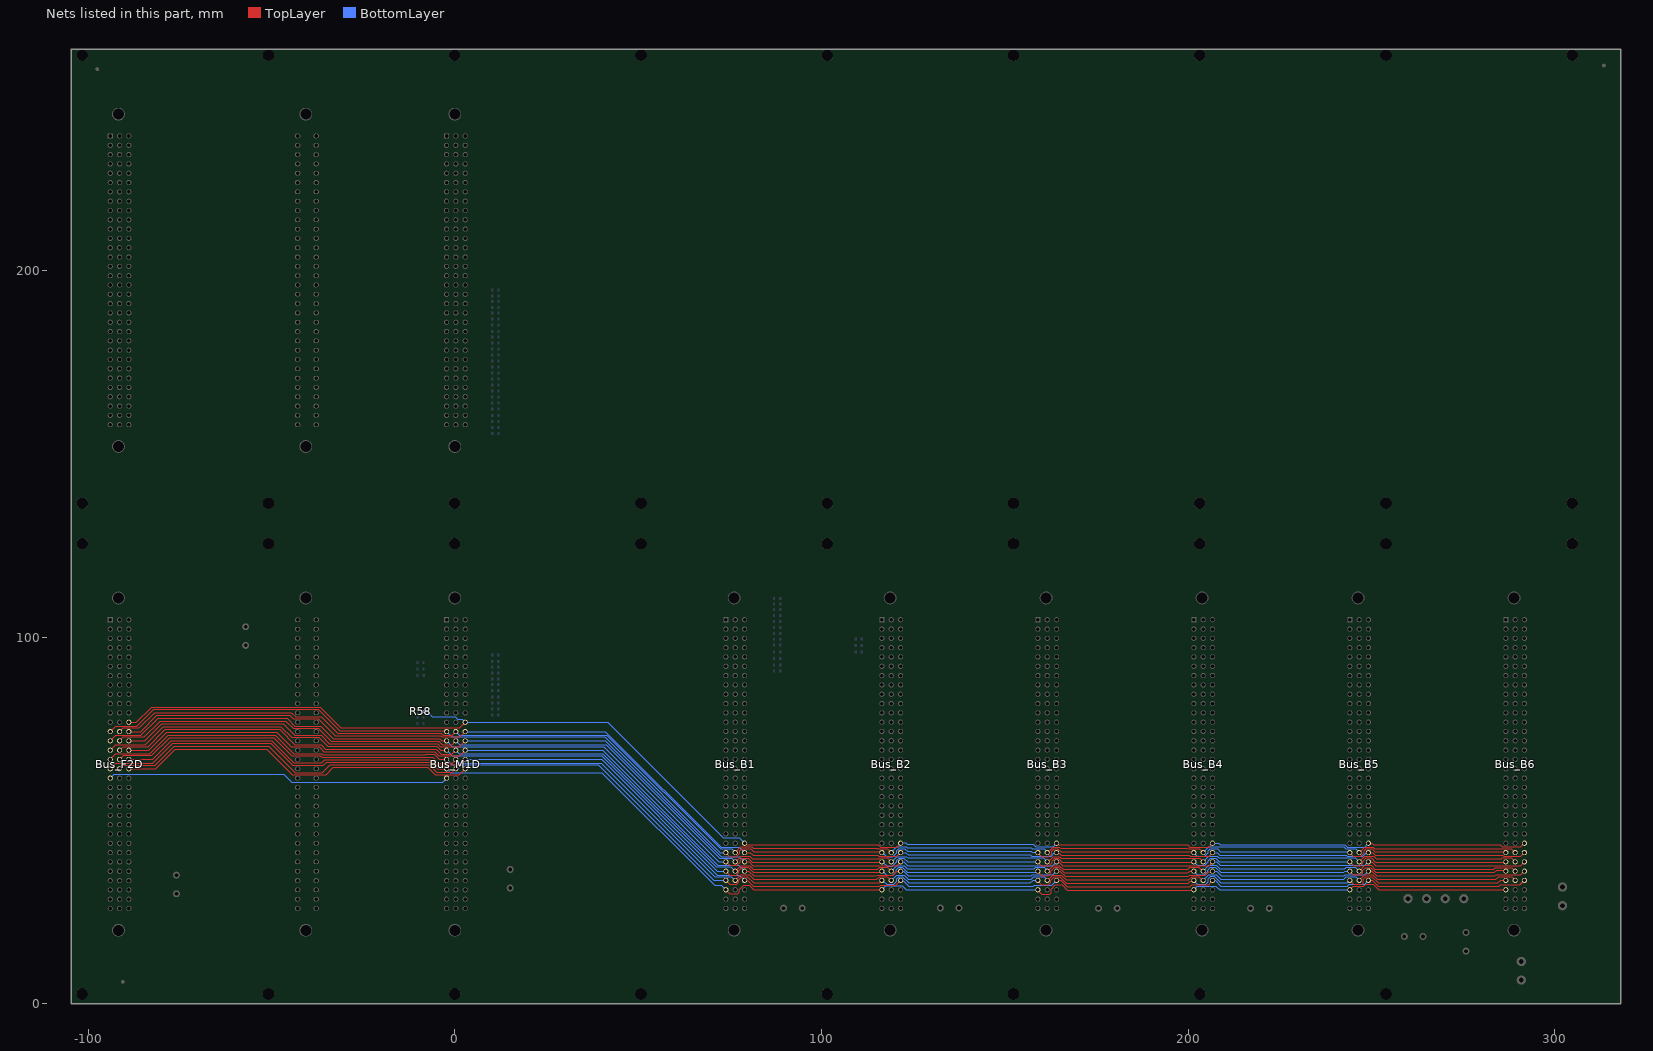
[diagram p0: the nets of this part, all layers, seen from the top]
# Altium PCB MISC67337.PcbDoc (part 2 of 7)
Units mm, origin at the board's own origin, x right, y up, seen from the top; angles counter-clockwise.
Board outline 422.71 x 260.35 mm, 4 copper layers (TopLayer, InternalPlane1, InternalPlane2, BottomLayer); 82 components, 143 nets, 1295 pads, 42 vias.

## Via types
v1: diameter 0.61, hole 0.305, TopLayer to BottomLayer, 42 vias

## Nets (pads, with @x,y where several pads share a name; then routed paths per layer and width w, separated by ;. In a path a pad name is that pad's centre, name@x,y a point inside that pad or via, vN(x,y) a via of type N, cw(c..) or ccw(c..) an arc to the next point about the centre after c; other vN are vias at no path point) (continued)
B_DSP1_X\W\E\: Bus_B1.C25 Bus_B2.C25 Bus_B3.C25 Bus_B4.C25 Bus_B5.C25 Bus_B6.C25 Bus_F2D.C12 Bus_M1D.C12 R58.2 | length 420.3
  TopLayer w0.254: Bus_F2D.C12@-88.89,76.754 -86.822,76.754 -82.68,80.896 -36.7,80.896 -31.039,75.235 1.321,75.235 Bus_M1D.C12@2.84,76.754 ; Bus_B1.C25@79.04,43.324 113.233,43.324 ; 113.727,43.324 113.233,43.324 ; Bus_B2.C25@121.521,43.817 Bus_B2.C25@121.585,43.88 ; Bus_B2.C25@121.585,43.753 120.504,42.672 116.203,42.672 115.551,43.324 113.233,43.324 ; Bus_B3.C25@164.13,43.308 198.425,43.308 ; 198.817,43.308 198.425,43.308 ; Bus_B4.C25@206.675,43.753 205.594,42.672 200.533,42.672 199.897,43.308 198.425,43.308 ; Bus_B5.C25@249.409,43.942 Bus_B5.C25@249.22,43.753 250.176,43.753 250.605,43.324 284.226,43.324 ; 284.607,43.324 284.226,43.324 ; Bus_B6.C25@291.765,43.753 290.787,42.775 285.774,42.775 285.225,43.324 284.226,43.324
  BottomLayer w0.254: R58.2@-8.484,79.705 -7.569,79.705 -6.18,78.316 0.121,78.316 0.84,77.597 1.997,77.597 Bus_M1D.C12@2.84,76.754 41.737,76.754 73.279,45.212 77.576,45.212 Bus_B1.C25@79.035,43.753 ; Bus_B2.C25@121.585,43.753 121.647,43.815 122.961,43.815 123.369,43.408 125.578,43.408 ; 124.93,43.408 125.578,43.408 ; 151.892,43.408 151.308,43.408 ; Bus_B3.C25@164.257,43.815 163.176,42.734 158.496,42.734 157.822,43.408 151.308,43.408 ; Bus_B4.C25@206.675,43.753 208.407,43.753 208.778,43.382 211.074,43.382 ; 209.893,43.382 211.074,43.382 ; 236.855,43.382 236.296,43.382 ; Bus_B5.C25@249.22,43.753 248.139,42.672 243.459,42.672 242.749,43.382 236.296,43.382 ; 125.578,43.408 151.308,43.408 ; 211.074,43.382 236.296,43.382
B_DSP1_XA0: Bus_B1.A26 Bus_B2.A26 Bus_B3.A26 Bus_B4.A26 Bus_B5.A26 Bus_B6.A26 Bus_F2D.A13 Bus_M1D.A13 | length 414.4
  TopLayer w0.254: Bus_F2D.A13@-93.97,74.214 -92.492,75.692 -86.69,75.692 -82.118,80.264 -37.236,80.264 -31.411,74.438 Bus_M1D.A13@-2.6,74.438 ; Bus_M1D.A13@-2.6,74.574 Bus_M1D.A13@-2.24,74.214 ; Bus_B1.A26@73.96,41.213 75.041,40.132 76.835,40.132 77.724,41.021 77.724,41.656 78.259,42.191 80.779,42.191 81.534,41.436 112.243,41.436 ; 113.349,41.436 112.243,41.436 ; Bus_B2.A26@116.505,41.213 Bus_B2.A26@116.378,41.34 ; Bus_B2.A26@116.505,41.34 Bus_B2.A26@116.378,41.34 ; Bus_B3.A26@159.05,41.086 160.131,40.005 161.925,40.005 162.814,40.894 162.814,41.529 163.576,42.291 164.491,42.291 165.379,41.403 197.993,41.403 ; 198.439,41.403 197.993,41.403 ; Bus_B4.A26@201.595,41.086 201.468,41.213 Bus_B4.A26@201.595,41.213 201.405,41.403 197.993,41.403 ; Bus_B5.A26@244.14,41.213 245.118,40.235 247.118,40.235 248.031,41.148 248.031,41.656 248.566,42.191 250.188,42.191 250.943,41.436 286.462,41.436 Bus_B6.A26@286.685,41.213 ; 112.243,41.436 116.282,41.436 Bus_B2.A26@116.378,41.34
  BottomLayer w0.254: Bus_M1D.A13@-2.24,74.214 -0.797,72.771 40.894,72.771 72.452,41.213 Bus_B1.A26@73.955,41.213 ; Bus_B2.A26@116.632,41.275 117.775,40.132 119.445,40.132 120.523,41.21 120.523,41.718 121.071,42.266 122.758,42.266 123.517,41.507 154.584,41.507 ; 156.424,41.507 154.584,41.507 ; Bus_B3.A26@159.177,41.275 157.415,41.275 157.183,41.507 154.584,41.507 ; Bus_B4.A26@201.595,41.213 202.573,40.235 204.573,40.235 205.486,41.148 205.486,41.656 206.045,42.215 208.077,42.215 208.807,41.485 240.208,41.485 ; 241.222,41.485 240.208,41.485 ; Bus_B5.A26@244.14,41.213 243.868,41.485 240.208,41.485
B_DSP1_XA1: Bus_B1.B26 Bus_B2.B26 Bus_B3.B26 Bus_B4.B26 Bus_B5.B26 Bus_B6.B26 Bus_F2D.B13 Bus_M1D.B13 | length 408.8
  TopLayer w0.254: Bus_F2D.B13@-91.43,74.214 -90.452,75.192 -85.996,75.192 -81.819,79.369 -44.571,79.369 -43.434,78.232 -36.449,78.232 -31.941,73.724 -3.632,73.724 -3.144,73.236 -0.678,73.236 Bus_M1D.B13@0.3,74.214 ; Bus_B1.B26@76.495,41.213 78.057,42.775 80.961,42.775 81.356,42.38 115.328,42.38 115.443,42.266 ; 115.418,42.266 115.443,42.266 ; Bus_B2.B26@119.045,41.213 117.992,42.266 115.443,42.266 ; Bus_B3.B26@161.59,41.086 163.201,42.697 164.885,42.697 165.227,42.355 198.857,42.355 ; 199.011,42.355 198.857,42.355 ; Bus_B4.B26@204.135,41.086 203.03,42.191 199.998,42.191 199.834,42.355 198.857,42.355 ; Bus_B5.B26@246.68,41.213 246.699,41.213 248.158,42.672 250.508,42.672 250.889,42.291 285.826,42.291 ; 285.115,42.291 285.826,42.291 ; Bus_B6.B26@289.225,41.213 288.147,42.291 285.826,42.291
  BottomLayer w0.254: Bus_M1D.B13@0.3,74.214 1.278,73.236 41.443,73.236 72.488,42.191 75.517,42.191 Bus_B1.B26@76.495,41.213 ; Bus_B2.B26@119.045,41.213 120.58,42.748 123.178,42.748 123.469,42.457 125.527,42.457 155.169,42.457 ; 157.161,42.457 155.169,42.457 ; Bus_B3.B26@161.717,41.275 160.739,42.253 157.493,42.253 157.288,42.457 155.169,42.457 ; Bus_B4.B26@204.135,41.213 205.67,42.748 242.494,42.748 243.051,42.191 245.702,42.191 Bus_B5.B26@246.68,41.213
B_DSP1_XA2: Bus_B1.C26 Bus_B2.C26 Bus_B3.C26 Bus_B4.C26 Bus_B5.C26 Bus_B6.C26 Bus_F2D.C13 Bus_M1D.C13 | length 408.7
  TopLayer w0.254: Bus_F2D.C13@-88.89,74.214 -85.704,74.214 -81.313,78.606 -45.027,78.606 -44.09,77.668 -37.257,77.668 -32.599,73.01 -6.096,73.01 ; -3.835,73.01 -6.096,73.01 ; Bus_M1D.C13@2.84,74.214 1.397,72.771 -3.581,72.771 -3.82,73.01 -6.096,73.01 ; Bus_B1.C26@79.035,41.213 Bus_B1.C26@79.04,41.213 ; Bus_B1.C26@79.229,41.402 Bus_B1.C26@79.04,41.213 ; Bus_B2.C26@121.585,41.213 120.529,40.157 115.672,40.157 115.337,40.492 81.377,40.492 80.656,41.213 Bus_B1.C26@79.04,41.213 ; Bus_B3.C26@164.13,41.086 Bus_B3.C26@164.193,41.15 ; Bus_B3.C26@164.13,41.213 Bus_B3.C26@164.193,41.15 ; Bus_B3.C26@164.319,41.275 Bus_B3.C26@164.193,41.15 ; Bus_B4.C26@206.675,41.086 205.746,40.157 200.635,40.157 200.342,40.45 165.467,40.45 164.768,41.15 Bus_B3.C26@164.193,41.15 ; Bus_B5.C26@249.22,41.213 250.404,41.213 251.125,40.492 283.718,40.492 ; 284.034,40.492 283.718,40.492 ; 286.106,40.235 286.131,40.235 ; Bus_B6.C26@291.765,41.213 290.787,40.235 286.131,40.235 ; 283.718,40.492 285.874,40.492 286.131,40.235
  BottomLayer w0.254: Bus_M1D.C13@2.84,74.214 41.102,74.214 72.644,42.672 77.576,42.672 Bus_B1.C26@79.035,41.213 ; Bus_B2.C26@121.585,41.213 123.023,41.213 123.68,40.557 155.6,40.557 ; 156.272,40.557 155.6,40.557 ; Bus_B3.C26@164.257,41.275 163.673,41.275 162.631,40.234 157.313,40.234 156.99,40.557 155.6,40.557 ; Bus_B4.C26@206.675,41.213 208.012,41.213 208.688,40.537 239.776,40.537 ; 241.235,40.537 239.776,40.537 ; Bus_B5.C26@249.22,41.213 248.636,41.213 247.658,40.235 243.434,40.235 243.132,40.537 239.776,40.537
B_DSP1_XA3: Bus_B1.A27 Bus_B2.A27 Bus_B3.A27 Bus_B4.A27 Bus_B5.A27 Bus_B6.A27 Bus_F2D.A14 Bus_M1D.A14 | length 415.5
  TopLayer w0.254: Bus_F2D.A14@-93.97,71.674 -92.492,73.152 -85.623,73.152 -80.933,77.842 -45.736,77.842 -43.586,75.692 -36.601,75.692 -33.205,72.296 -6.426,72.296 ; -4.496,72.296 -6.426,72.296 ; Bus_M1D.A14@-2.24,71.674 -3.526,71.674 -4.148,72.296 -6.426,72.296 ; Bus_B1.A27@73.96,38.673 74.938,37.695 76.938,37.695 77.851,38.608 77.851,39.116 78.386,39.651 80.085,39.651 81.131,38.604 113.665,38.604 ; 113.944,38.604 113.665,38.604 ; Bus_B2.A27@116.505,38.673 116.436,38.604 113.665,38.604 ; Bus_B3.A27@159.05,38.546 160.028,37.568 162.028,37.568 162.941,38.481 162.941,38.989 163.603,39.651 164.641,39.651 165.747,38.546 198.069,38.546 ; 198.982,38.546 198.069,38.546 ; Bus_B4.A27@201.595,38.673 201.468,38.546 198.069,38.546 ; Bus_B5.A27@244.14,38.673 245.221,37.592 246.982,37.592 247.658,38.268 247.658,38.743 248.666,39.751 249.911,39.751 251.057,38.604 282.372,38.604 ; 283.34,38.604 282.372,38.604 ; Bus_B6.A27@286.685,38.673 286.616,38.604 282.372,38.604
  BottomLayer w0.254: Bus_M1D.A14@-2.24,71.674 -0.678,70.112 40.632,70.112 72.071,38.673 Bus_B1.A27@73.955,38.673 ; Bus_B2.A27@116.632,38.735 117.902,37.465 119.285,37.465 120.523,38.703 120.523,39.051 121.185,39.713 122.466,39.713 123.523,38.656 154.965,38.656 ; 155.929,38.656 154.965,38.656 ; Bus_B3.A27@159.05,38.673 159.033,38.656 154.965,38.656 ; Bus_B3.A27@159.05,38.735 Bus_B3.A27@159.177,38.735 ; Bus_B4.A27@201.595,38.673 202.573,37.695 204.54,37.695 205.486,38.641 205.486,38.989 206.148,39.651 207.567,39.651 208.578,38.64 240.005,38.64 ; 240.892,38.64 240.005,38.64 ; Bus_B5.A27@244.14,38.673 244.107,38.64 240.005,38.64
B_DSP1_XA4: Bus_B1.B27 Bus_B2.B27 Bus_B3.B27 Bus_B4.B27 Bus_B5.B27 Bus_B6.B27 Bus_F2D.B14 Bus_M1D.B14 | length 412.5
  TopLayer w0.254: Bus_F2D.B14@-91.43,71.674 -90.358,72.746 -84.684,72.746 -80.351,77.079 -46.065,77.079 -44.115,75.128 -37.232,75.128 -33.685,71.582 -29.642,71.582 ; -32.36,71.582 -29.642,71.582 ; -4.75,71.582 -5.817,71.582 ; Bus_M1D.B14@0.3,71.674 -0.751,70.623 -3.39,70.623 -4.348,71.582 -5.817,71.582 ; Bus_B1.B27@76.5,38.673 76.519,38.673 78.08,40.234 80.493,40.234 81.178,39.548 ; 81.153,39.548 81.178,39.548 ; 114.554,39.548 113.487,39.548 ; Bus_B2.B27@119.045,38.673 117.967,39.751 116.078,39.751 115.875,39.548 113.487,39.548 ; Bus_B3.B27@161.59,38.546 161.609,38.546 163.195,40.132 164.973,40.132 165.454,39.651 203.157,39.651 Bus_B4.B27@204.135,38.673 ; Bus_B4.B27@204.071,38.61 Bus_B4.B27@204.135,38.546 ; Bus_B5.B27@246.68,38.673 248.164,40.157 250.698,40.157 251.307,39.548 253.39,39.548 ; 252.425,39.548 253.39,39.548 ; 283.718,39.548 283.312,39.548 ; Bus_B6.B27@289.225,38.673 288.147,39.751 285.75,39.751 285.547,39.548 283.312,39.548 ; -29.642,71.582 -5.817,71.582 ; 81.178,39.548 113.487,39.548 ; 253.39,39.548 283.312,39.548
  BottomLayer w0.254: Bus_M1D.B14@0.3,71.674 1.362,70.612 41.275,70.612 72.236,39.651 75.517,39.651 Bus_B1.B27@76.495,38.673 ; Bus_B2.B27@119.172,38.735 120.569,40.132 123.139,40.132 123.546,39.726 160.537,39.726 Bus_B3.B27@161.59,38.673 ; Bus_B3.B27@161.684,38.768 Bus_B3.B27@161.717,38.735 ; Bus_B4.B27@204.135,38.673 205.645,40.183 207.924,40.183 208.356,39.751 245.602,39.751 Bus_B5.B27@246.68,38.673
B_DSP1_XA5: Bus_B1.C27 Bus_B2.C27 Bus_B3.C27 Bus_B4.C27 Bus_B5.C27 Bus_B6.C27 Bus_F2D.C14 Bus_M1D.C14 | length 410.1
  TopLayer w0.254: Bus_F2D.C14@-88.89,71.674 -84.557,71.674 -79.929,76.302 ; -79.929,76.315 -46.749,76.315 -43.586,73.152 -36.474,73.152 -34.19,70.867 -32.36,70.867 ; -33.249,70.867 -32.36,70.867 ; -5.174,70.867 -5.664,70.867 ; Bus_M1D.C14@2.84,71.674 1.278,70.112 -3.937,70.112 -4.693,70.867 -5.664,70.867 ; Bus_B1.C27@79.035,38.673 Bus_B1.C27@79.04,38.673 ; Bus_B1.C27@79.356,38.989 Bus_B1.C27@79.04,38.673 ; 113.538,37.661 112.674,37.661 ; Bus_B2.C27@121.585,38.673 120.573,37.661 112.674,37.661 ; Bus_B3.C27@164.13,38.546 Bus_B3.C27@164.257,38.673 ; Bus_B3.C27@164.13,38.673 Bus_B3.C27@164.257,38.673 ; Bus_B3.C27@164.446,38.862 Bus_B3.C27@164.257,38.673 ; 198.628,37.593 198.095,37.593 ; 199.873,37.617 200.99,37.617 ; Bus_B4.C27@206.675,38.546 205.746,37.617 200.99,37.617 ; Bus_B5.C27@249.22,38.673 250.125,38.673 251.137,37.661 282.448,37.661 ; 282.829,37.661 282.448,37.661 ; Bus_B6.C27@291.765,38.673 290.753,37.661 282.448,37.661 ; -32.36,70.867 -5.664,70.867 ; Bus_B1.C27@79.04,38.673 80.301,38.673 81.313,37.661 112.674,37.661 ; Bus_B3.C27@164.257,38.673 164.73,38.673 165.81,37.593 198.095,37.593 ; 198.095,37.593 198.119,37.617 200.99,37.617
  BottomLayer w0.254: Bus_M1D.C14@2.84,71.674 41.102,71.674 72.644,40.132 77.576,40.132 Bus_B1.C27@79.035,38.673 ; Bus_B2.C27@121.585,38.673 122.515,38.673 123.546,37.643 163.1,37.643 Bus_B3.C27@164.13,38.673 ; Bus_B3.C27@164.163,38.641 Bus_B3.C27@164.257,38.735 ; Bus_B4.C27@206.675,38.673 207.783,38.673 208.765,37.691 239.573,37.691 ; 240.73,37.691 239.573,37.691 ; Bus_B5.C27@249.22,38.673 248.238,37.691 239.573,37.691
B_DSP1_XA6: Bus_B1.A28 Bus_B2.A28 Bus_B3.A28 Bus_B4.A28 Bus_B5.A28 Bus_B6.A28 Bus_F2D.A15 Bus_M1D.A15 | length 424.1
  TopLayer w0.254: Bus_F2D.A15@-93.97,69.134 -92.492,70.612 -84.404,70.612 ; -79.604,75.413 -84.404,70.612 ; -33.503,70.153 -31.521,70.153 ; -5.334,70.153 -6.858,70.153 ; Bus_M1D.A15@-2.24,69.134 -3.881,69.134 -4.901,70.153 -6.858,70.153 ; Bus_B1.A28@73.96,36.133 75.041,35.052 76.802,35.052 77.478,35.728 77.478,36.203 78.435,37.16 80.061,37.16 81.448,35.773 111.658,35.773 ; 112.398,35.773 111.658,35.773 ; Bus_B2.A28@116.505,36.133 116.145,35.773 111.658,35.773 ; Bus_B3.A28@159.05,36.006 160.131,34.925 161.892,34.925 162.568,35.601 162.568,36.076 163.703,37.211 164.668,37.211 166.191,35.688 197.256,35.688 ; 197.488,35.688 197.256,35.688 ; Bus_B4.A28@201.595,36.133 200.406,36.133 199.961,35.688 197.256,35.688 ; Bus_B5.A28@244.14,36.133 245.118,35.155 247.085,35.155 247.658,35.728 247.658,36.33 248.439,37.111 249.833,37.111 251.171,35.773 283.55,35.773 284.226,36.449 286.369,36.449 Bus_B6.A28@286.685,36.133 ; -84.404,70.612 -79.465,75.552 -47.408,75.552 -44.501,72.644 -37.135,72.644 -34.644,70.153 -31.521,70.153 ; -31.521,70.153 -6.858,70.153
  BottomLayer w0.254: Bus_M1D.A15@-2.24,69.134 -0.678,67.572 40.124,67.572 71.563,36.133 Bus_B1.A28@73.955,36.133 ; Bus_B2.A28@116.632,36.195 117.775,35.052 119.445,35.052 120.396,36.003 120.396,36.511 121.058,37.173 122.06,37.173 123.428,35.805 154.635,35.805 ; 155.04,35.805 154.635,35.805 ; Bus_B3.A28@159.177,36.195 158.988,36.195 Bus_B3.A28@159.05,36.133 158.722,35.805 154.635,35.805 ; Bus_B4.A28@201.595,36.133 202.573,35.155 204.573,35.155 205.359,35.941 205.359,36.449 206.07,37.16 207.493,37.16 208.858,35.795 239.319,35.795 ; 240.003,35.795 239.319,35.795 ; Bus_B5.A28@244.14,36.133 242.849,36.133 242.511,35.795 239.319,35.795
B_DSP1_XA7: Bus_B1.B28 Bus_B2.B28 Bus_B3.B28 Bus_B4.B28 Bus_B5.B28 Bus_B6.B28 Bus_F2D.B15 Bus_M1D.B15 | length 414.1
  TopLayer w0.254: Bus_F2D.B15@-91.43,69.134 -90.452,70.112 -83.668,70.112 -78.991,74.788 -47.788,74.788 -43.612,70.612 -36.474,70.612 -35.302,69.439 -7.595,69.439 ; -5.486,69.439 -7.595,69.439 ; Bus_M1D.B15@0.3,69.134 -0.762,68.072 -3.708,68.072 -5.076,69.439 -7.595,69.439 ; Bus_B1.B28@76.5,36.133 78.035,37.668 80.467,37.668 81.419,36.717 115.406,36.717 115.875,37.186 117.992,37.186 Bus_B2.B28@119.045,36.133 ; Bus_B3.B28@161.59,36.006 163.252,37.668 164.922,37.668 165.95,36.641 198.018,36.641 ; 198.222,36.641 198.018,36.641 ; Bus_B4.B28@204.135,36.006 202.93,37.211 200.533,37.211 199.963,36.641 198.018,36.641 ; Bus_B5.B28@246.68,36.133 248.242,37.695 249.934,37.695 250.913,36.717 282.981,36.717 ; 283.234,36.717 282.981,36.717 ; Bus_B6.B28@289.225,36.133 288.247,37.111 283.818,37.111 283.424,36.717 282.981,36.717
  BottomLayer w0.254: Bus_M1D.B15@0.3,69.134 1.278,68.156 40.429,68.156 71.296,37.289 75.339,37.289 Bus_B1.B28@76.495,36.133 ; Bus_B2.B28@119.172,36.195 120.569,37.592 122.555,37.592 123.392,36.755 154.051,36.755 ; 155.637,36.755 154.051,36.755 ; Bus_B3.B28@161.717,36.195 160.777,37.135 158.471,37.135 158.091,36.755 154.051,36.755 ; Bus_B4.B28@204.135,36.133 205.697,37.695 207.643,37.695 208.595,36.743 238.684,36.743 ; 240.435,36.743 238.684,36.743 ; Bus_B5.B28@246.68,36.133 245.602,37.211 243.205,37.211 242.737,36.743 238.684,36.743
B_DSP1_XA8: Bus_B1.C28 Bus_B2.C28 Bus_B3.C28 Bus_B4.C28 Bus_B5.C28 Bus_B6.C28 Bus_F2D.C15 Bus_M1D.C15 | length 413.3
  TopLayer w0.254: Bus_F2D.C15@-88.89,69.134 -83.469,69.134 -78.579,74.025 -48.523,74.025 -44.547,70.048 -37.003,70.048 -35.68,68.725 -31.572,68.725 ; -34.62,68.725 -31.572,68.725 ; -5.664,68.725 -6.68,68.725 ; Bus_M1D.C15@2.84,69.134 1.372,67.666 -4.369,67.666 -5.428,68.725 -6.68,68.725 ; Bus_B1.C28@79.035,36.133 80.199,36.133 81.503,34.829 83.718,34.829 ; 82.652,34.829 83.718,34.829 ; 111.887,34.829 111.658,34.829 ; Bus_B2.C28@121.585,36.133 120.588,36.133 119.532,35.077 115.214,35.077 114.966,34.829 111.658,34.829 ; Bus_B3.C28@164.13,36.133 165.06,36.133 166.458,34.736 196.799,34.736 ; 196.977,34.736 196.799,34.736 ; Bus_B4.C28@206.675,36.006 205.678,36.006 204.749,35.077 200.431,35.077 200.09,34.736 196.799,34.736 ; Bus_B5.C28@249.22,36.133 250.15,36.133 251.455,34.829 282.296,34.829 ; 282.764,34.829 282.296,34.829 ; Bus_B6.C28@291.765,36.133 290.787,35.155 284.024,35.155 283.698,34.829 282.296,34.829 ; -31.572,68.725 -6.68,68.725 ; 83.718,34.829 111.658,34.829
  BottomLayer w0.254: Bus_M1D.C15@2.84,69.134 40.34,69.134 71.779,37.695 77.473,37.695 Bus_B1.C28@79.035,36.133 ; Bus_B2.C28@121.585,36.133 122.439,36.133 123.718,34.854 154.407,34.854 ; 155.002,34.854 154.407,34.854 ; Bus_B3.C28@164.257,36.195 163.165,35.103 157.556,35.103 157.308,34.854 154.407,34.854 ; Bus_B4.C28@206.675,36.133 207.783,36.133 209.07,34.846 238.404,34.846 ; 239.965,34.846 238.404,34.846 ; Bus_B5.C28@249.22,36.133 248.242,35.155 242.862,35.155 242.553,34.846 238.404,34.846
B_DSP1_XA9: Bus_B1.A29 Bus_B2.A29 Bus_B3.A29 Bus_B4.A29 Bus_B5.A29 Bus_B6.A29 Bus_F2D.A16 Bus_M1D.A16 | length 420.3
  TopLayer w0.254: Bus_F2D.A16@-93.97,66.594 -92.408,68.156 -83.202,68.156 -78.098,73.261 -49.004,73.261 -43.899,68.156 -36.228,68.156 -35.941,67.869 -7.889,67.869 -7.747,68.011 ; -6.198,68.011 -7.747,68.011 ; Bus_M1D.A16@-2.24,66.594 -4.212,66.594 -5.628,68.011 -7.747,68.011 ; Bus_B1.A29@73.96,33.593 74.938,32.615 76.905,32.615 77.478,33.188 77.478,33.79 78.334,34.646 79.832,34.646 81.537,32.941 82.55,32.941 ; 82.269,32.941 82.55,32.941 ; Bus_B2.A29@116.505,33.593 115.853,32.941 82.55,32.941 ; Bus_B3.A29@159.05,33.466 160.028,32.488 161.995,32.488 162.568,33.061 162.568,33.663 163.476,34.571 165.073,34.571 166.813,32.831 170.383,32.831 ; 167.359,32.831 170.383,32.831 ; Bus_B4.A29@201.595,33.466 Bus_B4.A29@201.468,33.466 ; Bus_B4.A29@201.595,33.593 Bus_B4.A29@201.468,33.466 ; Bus_B5.A29@244.14,33.593 245.221,32.512 247.396,32.512 247.777,32.893 247.777,33.909 248.539,34.671 250.139,34.671 251.869,32.941 281.864,32.941 ; 282.067,32.941 281.864,32.941 ; Bus_B6.A29@286.685,33.593 286.572,33.706 285.267,33.706 284.502,32.941 281.864,32.941 ; 170.383,32.831 200.115,32.831 200.609,33.325 201.327,33.325 Bus_B4.A29@201.468,33.466
  BottomLayer w0.254: Bus_M1D.A16@-2.24,66.594 -0.797,65.151 39.116,65.151 70.674,33.593 Bus_B1.A29@73.955,33.593 ; Bus_B2.A29@116.632,33.655 117.775,32.512 119.699,32.512 120.523,33.336 120.523,34.098 121.071,34.646 122.098,34.646 123.79,32.954 153.137,32.954 ; 153.973,32.954 153.137,32.954 ; Bus_B3.A29@159.05,33.593 Bus_B3.A29@158.988,33.655 ; Bus_B3.A29@159.177,33.655 Bus_B3.A29@158.988,33.655 ; Bus_B4.A29@201.595,33.593 202.573,32.615 204.827,32.615 205.486,33.274 205.486,34.036 206.199,34.749 207.135,34.749 208.934,32.95 238.455,32.95 ; 238.936,32.95 238.455,32.95 ; Bus_B5.A29@244.14,33.593 243.497,32.95 238.455,32.95 ; 153.137,32.954 157.033,32.954 157.734,33.655 Bus_B3.A29@158.988,33.655
B_DSP1_XA10: Bus_B1.B29 Bus_B2.B29 Bus_B3.B29 Bus_B4.B29 Bus_B5.B29 Bus_B6.B29 Bus_F2D.B16 Bus_M1D.B16 | length 413.9
  TopLayer w0.254: Bus_F2D.B16@-91.43,66.594 -90.333,67.691 -82.601,67.691 -77.794,72.498 -49.409,72.498 -44.491,67.58 -36.643,67.58 -36.322,67.259 -5.994,67.259 -4.351,65.616 -0.678,65.616 Bus_M1D.B16@0.3,66.594 ; Bus_B1.B29@76.5,33.593 78.062,35.155 80.339,35.155 81.609,33.885 83.109,33.885 ; 81.915,33.885 83.109,33.885 ; 111.633,33.885 111.455,33.885 ; Bus_B2.B29@119.045,33.593 117.967,34.671 115.951,34.671 115.165,33.885 111.455,33.885 ; Bus_B3.B29@161.59,33.466 163.152,35.028 165.479,35.028 166.724,33.783 200.255,33.783 201.143,34.671 202.93,34.671 Bus_B4.B29@204.135,33.466 ; Bus_B5.B29@246.68,33.593 248.242,35.155 250.366,35.155 251.637,33.885 282.092,33.885 ; 282.575,33.885 282.092,33.885 ; Bus_B6.B29@289.225,33.593 288.247,34.571 284.685,34.571 283.999,33.885 282.092,33.885 ; 83.109,33.885 111.455,33.885
  BottomLayer w0.254: Bus_M1D.B16@0.3,66.594 1.337,65.557 39.98,65.557 70.866,34.671 75.417,34.671 Bus_B1.B29@76.495,33.593 ; Bus_B2.B29@119.172,33.655 120.569,35.052 121.952,35.052 122.58,35.052 123.728,33.904 154.153,33.904 ; 154.686,33.904 154.153,33.904 ; Bus_B3.B29@161.717,33.655 160.777,34.595 157.886,34.595 157.196,33.904 154.153,33.904 ; Bus_B4.B29@204.135,33.593 205.697,35.155 207.72,35.155 208.977,33.898 237.541,33.898 ; 239.649,33.898 237.541,33.898 ; Bus_B5.B29@246.68,33.593 245.702,34.571 243.129,34.571 242.456,33.898 237.541,33.898
B_DSP1_XA11: Bus_B1.C29 Bus_B2.C29 Bus_B3.C29 Bus_B4.C29 Bus_B5.C29 Bus_B6.C29 Bus_F2D.C16 Bus_M1D.C16 | length 413.7
  TopLayer w0.254: Bus_F2D.C16@-88.89,66.594 -82.402,66.594 -77.262,71.734 -49.915,71.734 -43.861,65.68 -43.277,65.68 ; -43.256,65.659 -36.322,65.659 -35.399,66.582 -8.484,66.582 ; -6.477,66.582 -8.484,66.582 ; Bus_M1D.C16@2.84,66.594 1.397,65.151 -4.826,65.151 -6.257,66.582 -8.484,66.582 ; Bus_B1.C29@79.035,33.593 79.818,33.593 81.414,31.997 110.744,31.997 ; 111.125,31.997 110.744,31.997 ; Bus_B2.C29@121.585,33.593 120.25,32.258 116.129,32.258 115.868,31.997 110.744,31.997 ; Bus_B3.C29@164.13,33.593 165.34,33.593 167.054,31.878 167.996,31.878 ; 167.767,31.878 167.996,31.878 ; 196.215,31.878 195.859,31.878 ; Bus_B4.C29@206.675,33.466 205.697,32.488 201.016,32.488 200.406,31.878 195.859,31.878 ; Bus_B5.C29@249.536,33.909 Bus_B5.C29@249.22,33.593 250.252,33.593 251.848,31.997 284.803,31.997 285.166,32.36 290.532,32.36 Bus_B6.C29@291.765,33.593 290.684,32.512 ; 167.996,31.878 195.859,31.878
  BottomLayer w0.254: Bus_M1D.C16@2.84,66.594 40.086,66.594 71.603,35.077 77.551,35.077 Bus_B1.C29@79.035,33.593 ; Bus_B2.C29@121.585,33.593 122.211,33.593 123.8,32.003 157.733,32.003 158.013,32.283 162.82,32.283 Bus_B3.C29@164.13,33.593 ; Bus_B3.C29@164.163,33.561 Bus_B3.C29@164.257,33.655 ; Bus_B4.C29@207.118,34.036 Bus_B4.C29@206.675,33.593 207.402,33.593 208.994,32.001 237.515,32.001 ; 238.379,32.001 237.515,32.001 ; Bus_B5.C29@249.22,33.593 248.139,32.512 243.967,32.512 243.456,32.001 237.515,32.001
B_DSP1_XA12: Bus_B1.A30 Bus_B2.A30 Bus_B3.A30 Bus_B4.A30 Bus_B5.A30 Bus_B6.A30 Bus_F2D.A17 Bus_M1D.A17 | length 410.7
  TopLayer w0.254: Bus_F2D.A17@-93.97,64.054 -92.492,65.532 -82.398,65.532 -76.959,70.971 -75.209,70.971 ; -76.733,70.971 -75.209,70.971 ; -50.419,70.971 -50.825,70.971 ; Bus_M1D.A17@-2.24,64.054 -4.775,64.054 -6.589,65.868 -34.944,65.868 -35.844,64.968 -44.242,64.968 -50.244,70.971 -50.825,70.971 ; Bus_B1.A30@73.96,31.053 75.041,29.972 77.216,29.972 77.597,30.353 77.597,31.09 78.816,32.309 80.289,32.309 81.545,31.053 Bus_B2.A30@116.505,31.053 ; Bus_B3.A30@159.05,30.926 160.131,29.845 162.306,29.845 162.687,30.226 162.687,31.242 163.83,32.385 165.659,32.385 167.118,30.926 198.944,30.926 Bus_B4.A30@201.595,30.926 ; Bus_B5.A30@244.14,31.053 245.118,32.031 247.931,32.031 248.463,32.563 250.571,32.563 252.081,31.053 Bus_B6.A30@286.685,31.053 ; -75.209,70.971 -50.825,70.971
  BottomLayer w0.254: Bus_M1D.A17@-2.24,64.054 -1.178,62.992 40.132,62.992 70.866,32.258 72.75,32.258 Bus_B1.A30@73.955,31.053 ; Bus_B2.A30@116.632,31.115 117.61,32.093 122.074,32.093 123.114,31.053 124.816,31.053 Bus_B3.A30@159.05,31.053 ; Bus_B3.A30@159.05,31.115 Bus_B3.A30@159.177,31.115 ; Bus_B4.A30@201.595,31.053 202.573,32.031 207.618,32.031 208.596,31.053 Bus_B5.A30@244.14,31.053
B_DSP1_XA13: Bus_F2D.B17 Bus_M1D.B17 | length 99.4
  TopLayer w0.254: Bus_F2D.B17@-91.43,64.054 -90.452,65.032 -81.653,65.032 -76.478,70.207 -50.725,70.207 -43.51,62.992 -36.246,62.992 -36.093,62.992 -33.931,65.154 -32.41,65.154 -6.937,65.154 -4.859,63.076 -0.678,63.076 Bus_M1D.B17@0.3,64.054
B_DSP1_XA14: Bus_F2D.C17 Bus_M1D.C17 | length 99.2
  TopLayer w0.254: Bus_F2D.C17@-88.89,64.054 -81.559,64.054 -76.17,69.444 -51.283,69.444 -44.298,62.459 -35.077,62.459 -33.096,64.44 -7.366,64.44 -5.385,62.459 -2.678,62.459 -2.645,62.492 1.278,62.492 Bus_M1D.C17@2.84,64.054
B_DSP1_XA15: Bus_F2D.A18 Bus_M1D.A18 | length 93.5
  BottomLayer w0.254: Bus_F2D.A18@-93.97,61.514 -92.873,62.611 -46.711,62.611 -44.526,60.427 -3.327,60.427 Bus_M1D.A18@-2.24,61.514